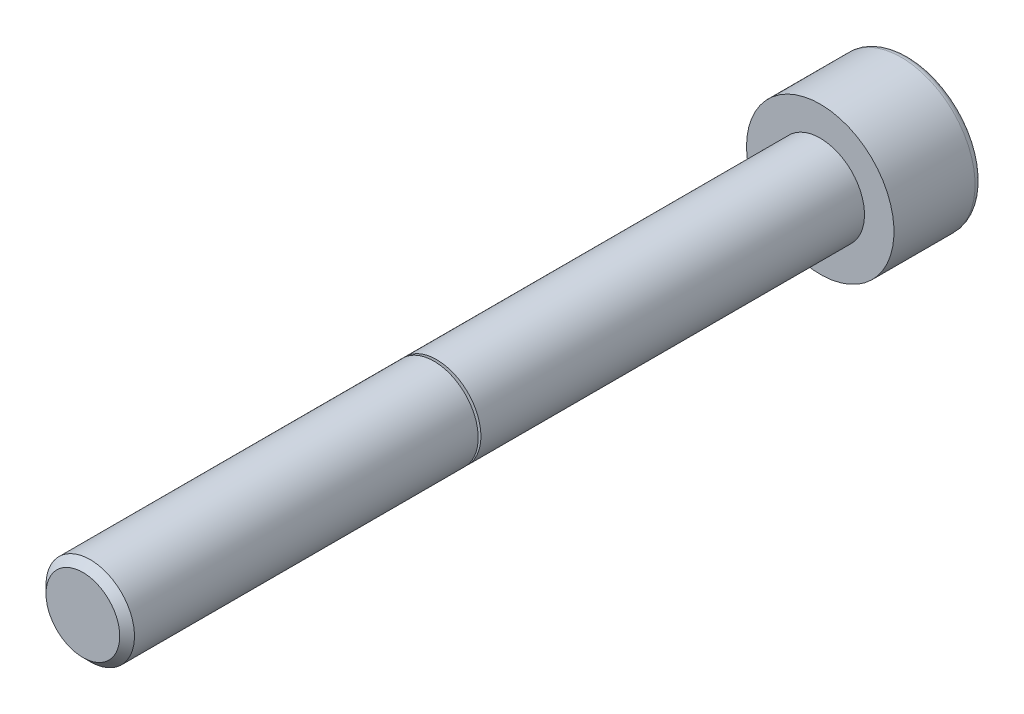
from build123d import *

# Parameters (mm, degrees)
CUT_EXTRUDE1_DEPTH = 2.5


with BuildPart() as part:
    # Logo3_bib1 → Revolve1 (revolve)
    with BuildSketch(Plane(origin=(0, 0, 0), x_dir=(-1, 0, 0), z_dir=(0, -1, 0))):
        with BuildLine():
            Line((0, -50), (0, 6))
            Line((0, 6), (4.5, 6))
            ThreePointArc((4.5, 6), (4.853553391, 5.853553391), (5, 5.5))
            Line((5, 5.5), (5, 0))
            Line((5, 0), (3, 0))
            Line((3, 0), (3, -26.01))
            Line((3, -26.01), (2.613425636, -26.01))
            ThreePointArc((2.613425636, -26.01), (2.593729481, -26.026527036), (2.606585234, -26.048793852))
            Line((2.606585234, -26.048793852), (3, -26.191985117))
            Line((3, -26.191985117), (3, -49.5))
            Line((3, -49.5), (2.5, -50))
            Line((2.5, -50), (0, -50))
        make_face()
    revolve(axis=Axis((0, 0, -10.585154653), (0, 0, 1)))

    # Logo3_bib2 → Cut-Extrude1 (cut)
    with BuildSketch(Plane(origin=(0, 0, -6), x_dir=(1, 0, 0), z_dir=(0, 0, -1))):
        Polygon((2.886751346, 0), (1.443375673, 2.5), (-1.443375673, 2.5), (-2.886751346, 0), (-1.443375673, -2.5), (1.443375673, -2.5), align=None)
    extrude(amount=-CUT_EXTRUDE1_DEPTH, mode=Mode.SUBTRACT)


solid = part.part
